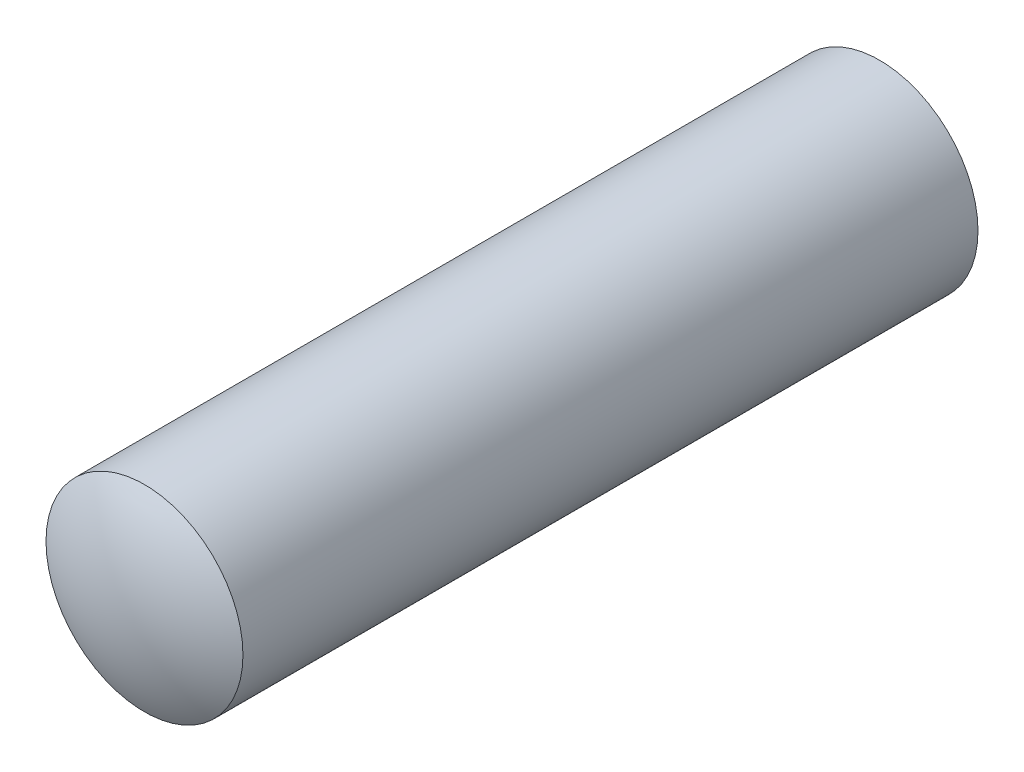
from build123d import *


with BuildPart() as part:
    # Logo3_bib1 → Revolve1 (revolve)
    with BuildSketch(Plane(origin=(0, 0, 0), x_dir=(-1, 0, 0), z_dir=(0, -1, 0))):
        with BuildLine():
            Line((0, 8), (0, -8))
            ThreePointArc((0, -8), (1.03527618, -7.863703305), (2, -7.464101615))
            Line((2, -7.464101615), (2, 7.464101615))
            ThreePointArc((2, 7.464101615), (1.03527618, 7.863703305), (0, 8))
        make_face()
    revolve(axis=Axis((0, 0, -47.537203702), (0, 0, 1)))


solid = part.part
